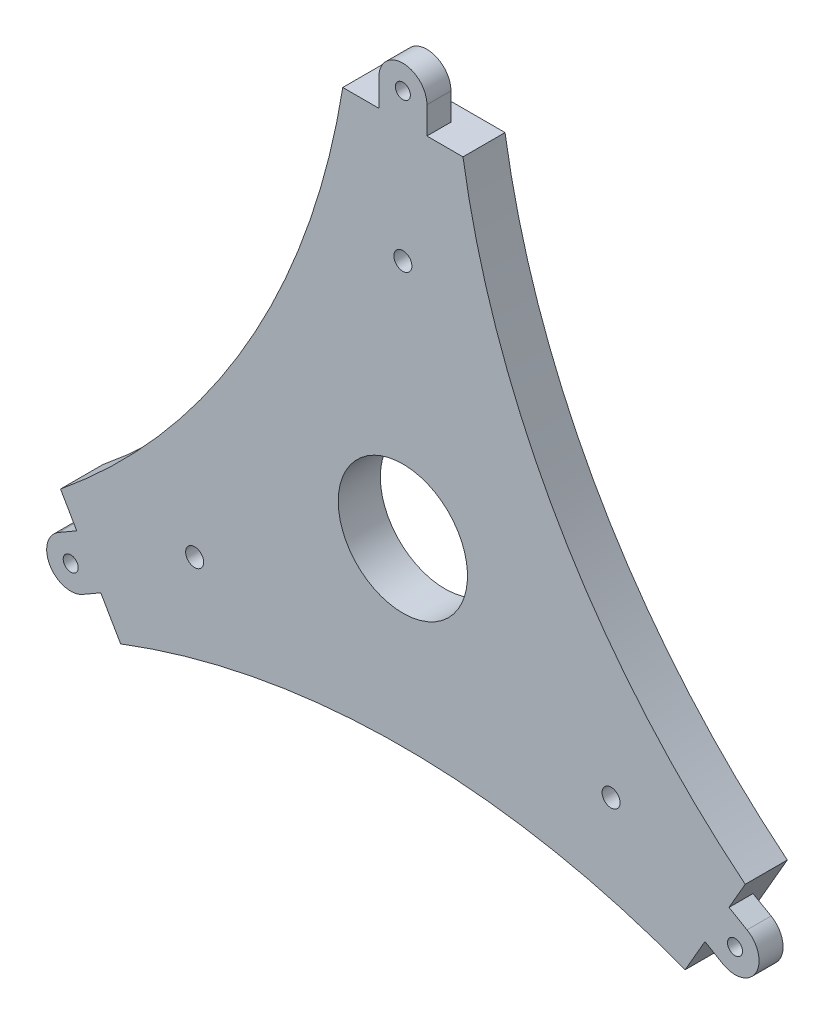
from build123d import *

# Parameters (mm, degrees)
BOSS_EXTRUDE1_DEPTH   = 14
BOSS_EXTRUDE2_DEPTH   = 8
CIRPATTERN1_COUNT     = 3
M6_TAPPED_HOLE1_D     = 5
M6_TAPPED_HOLE1_DEPTH = 15
M6_TAPPED_HOLE1_TIP   = 1.502151548
SKETCH5_R             = 21.5
CUT_EXTRUDE1_DEPTH    = 182.6949343
M6_TAPPED_HOLE2_D     = 5
M6_TAPPED_HOLE2_DEPTH = 15
M6_TAPPED_HOLE2_TIP   = 1.502151548
SKETCH7_R             = 3
CUT_EXTRUDE2_DEPTH    = 17


with BuildPart() as part:
    # Sketch2 → Boss-Extrude1 (new body)
    with BuildSketch(Plane.XY):
        with BuildLine():
            Line((-20, 120), (20, 120))
            ThreePointArc((20, 120), (51.961524227, 30), (113.923048454, -42.679491924))
            Line((113.923048454, -42.679491924), (93.923048454, -77.320508076))
            ThreePointArc((93.923048454, -77.320508076), (0, -60), (-93.923048454, -77.320508076))
            Line((-93.923048454, -77.320508076), (-113.923048454, -42.679491924))
            ThreePointArc((-113.923048454, -42.679491924), (-51.961524227, 30), (-20, 120))
        make_face()
    extrude(amount=BOSS_EXTRUDE1_DEPTH)

    # Sketch3 → Boss-Extrude2 (add)
    with BuildSketch(Plane.XY.offset(14)):
        with BuildLine():
            ThreePointArc((-8, 129), (0, 121), (8, 129))
            Line((8, 129), (-8, 129))
        make_face()
        with BuildLine():
            Line((-8, 129), (8, 129))
            ThreePointArc((8, 129), (0, 137), (-8, 129))
        make_face()
        with BuildLine():
            ThreePointArc((-8, 129), (0, 121), (8, 129))
            Line((8, 129), (-8, 129))
        make_face()
        with BuildLine():
            Line((-8, 129), (8, 129))
            ThreePointArc((8, 129), (0, 137), (-8, 129))
        make_face()
        with BuildLine():
            Line((-8, 120), (8, 120))
            Line((8, 120), (8, 129))
            ThreePointArc((8, 129), (0, 121), (-8, 129))
            Line((-8, 129), (-8, 120))
        make_face()
    boss_extrude2 = extrude(amount=-BOSS_EXTRUDE2_DEPTH)

    # CirPattern1: Boss-Extrude2 ×3 about axis
    cirpattern1_axis = Axis((0, 1.377339071, 0), (0, 0, 1))
    for i in range(1, CIRPATTERN1_COUNT):
        add(boss_extrude2.rotate(cirpattern1_axis, i * 360 / CIRPATTERN1_COUNT))

    # M6 Tapped Hole1
    with Locations(Plane(origin=(0, 129, 6), x_dir=(-1, 0, 0), z_dir=(0, 0, -1))):
        with Locations((0, 0)):
            Hole(M6_TAPPED_HOLE1_D / 2, depth=M6_TAPPED_HOLE1_DEPTH)
            with Locations((0, 0, -(M6_TAPPED_HOLE1_DEPTH + M6_TAPPED_HOLE1_TIP / 2))):  # 118° drill point
                Cone(0, M6_TAPPED_HOLE1_D / 2, M6_TAPPED_HOLE1_TIP, mode=Mode.SUBTRACT)

    # Sketch5 → Cut-Extrude1 (cut, through all)
    with BuildSketch(Plane(origin=(0, 0, 0), x_dir=(-1, 0, 0), z_dir=(0, 0, -1))):
        Circle(SKETCH5_R)
    extrude(amount=-CUT_EXTRUDE1_DEPTH, mode=Mode.SUBTRACT)

    # M6 Tapped Hole2
    with Locations(Plane(origin=(-110.524466463, -62.433991393, 14), x_dir=(1, 0, 0), z_dir=(0, 0, 1))):
        with Locations((0, 0), (221.048932926, 0)):
            Hole(M6_TAPPED_HOLE2_D / 2, depth=M6_TAPPED_HOLE2_DEPTH)
            with Locations((0, 0, -(M6_TAPPED_HOLE2_DEPTH + M6_TAPPED_HOLE2_TIP / 2))):  # 118° drill point
                Cone(0, M6_TAPPED_HOLE2_D / 2, M6_TAPPED_HOLE2_TIP, mode=Mode.SUBTRACT)

    # Sketch7 → Cut-Extrude2 (cut)
    with BuildSketch(Plane(origin=(0, 0, 0), x_dir=(-1, 0, 0), z_dir=(0, 0, -1))):
        with Locations((0, 80)):
            Circle(SKETCH7_R)
        with Locations((69.282032303, -40)):
            Circle(SKETCH7_R)
        with Locations((-69.282032303, -40)):
            Circle(SKETCH7_R)
    extrude(amount=-CUT_EXTRUDE2_DEPTH, mode=Mode.SUBTRACT)


solid = part.part
